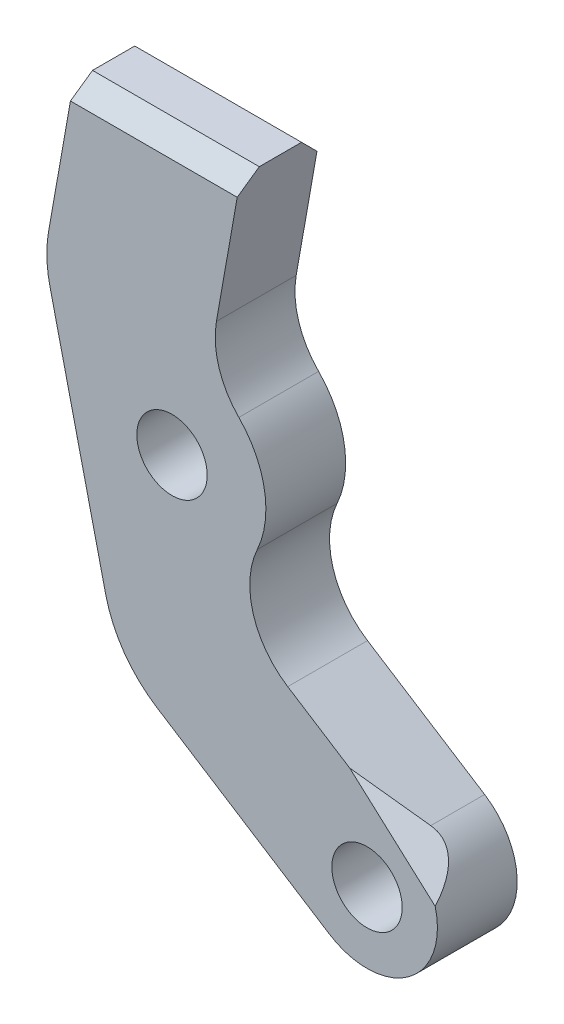
SolidWorks part; units mm, degrees
material "普通碳钢"
ref_plane "前视" through (0, 0, 0) normal (0, 0, 1) x (1, 0, 0)
ref_plane "上视" through (0, 0, 0) normal (0, 1, 0) x (1, 0, 0)
ref_plane "右视" through (0, 0, 0) normal (1, 0, 0) x (0, 0, -1)
sketch "草图1" plane through (0, 0, 0) normal (0, 0, 1) x (1, 0, 0)
  line L0 (-57.5777, 0) -> (30, 0) construction
  line L1 (0, 0) -> (0, -37.5217) construction
  line L2 (-125, 235) -> (-53.92, 235)
  line L3 (-125, 235) -> (-137.4861, 164.188)
  line L5 (-137.4861, 164.188) -> (-106.7282, 32.481)
  line L6 (-69.9882, 80.2135) -> (16.1306, 25.2944)
  line L8 (-106.7282, 32.481) -> (-16.1306, -25.2944)
  line L9 (50, 0) -> (-50, 0) construction
  line L10 (0, -50) -> (0, 50) construction
  line L12 (-53.92, 235) -> (-68.0184, 155.0438)
  arc A0 (-69.9882, 80.2135) -> (-58.4297, 86.5217) centre (-83.11, 118) ccw
  arc A2 (-58.4297, 86.5217) -> (-68.0184, 155.0438) centre (-83.11, 118) ccw
  arc A3 (-16.1306, -25.2944) -> (16.1306, 25.2944) centre (0, 0) ccw
  dimension "D10" = 53.92
  dimension "D7" = 164.188
  dimension "D4" = 30
  dimension "D5" = 40
  dimension "D2" = 235
  dimension "D3" = 70.0001
  dimension "D6" = 100
  dimension "D8" = 118
  dimension "D9" = 83.11
  dimension "D11" = 32.481
  dimension "D12" = 106.7282
  dimension "D13" = 137.4861
extrude "凸台-拉伸1" add sketch "草图1" along normal blind 34
chamfer "倒角1" distance 8 angle 45 2 edges at (-89.46, 235, 0) (-89.46, 235, 34)
sketch "草图2" plane through (0, 0, 0) normal (0, 0, -1) x (-1, 0, 0)
  line L1 (53.92, 235) -> (125, 235) construction
  line L2 (126.4106, 227) -> (137.4861, 164.188) construction
  line L3 (126.4106, 227) -> (137.4861, 164.188) construction
  circle A0 centre (0.0084, 0) radius 15
  circle A1 centre (83.1206, 118) radius 15
  dimension "D1" = 30
  dimension "D2" = 30
  dimension "D3" = 163.9
  dimension "D4" = 117
  dimension "D5" = 61.56
  dimension "D6" = 235
extrude "切除-拉伸1" cut sketch "草图2" against normal through all
fillet "圆角2" radius 35 2 edges at (-69.9882, 80.2135, 17) (-68.0184, 155.0438, 17)
fillet "圆角4" radius 50 2 edges at (-106.7282, 32.481, 17) (-137.4861, 164.188, 17)
ref_plane "基准面3" through (0, 0, 0) normal (0.7431, -0.6691, 0) x (0, 0, -1)
sketch "草图4" plane through (0, 0, 0) normal (0.7431, -0.6691, 0) x (0, 0, -1)
  line L0 (-34, 25) -> (-22, 30)
  line L1 (-34, 30) -> (-34, -29.5908) construction
  line L2 (-22, 30) -> (-34, 30)
  line L3 (-34, 43.966) -> (-34, 19.3666) construction
  line L4 (-34, 30) -> (-34, 25)
  line L5 (-34, 0) -> (0, 0) construction
  dimension "D1" = 5
  dimension "D2" = 12
  dimension "D3" = 25
extrude "切除-拉伸2" cut sketch "草图4" against normal up to surface and the other way through all up to face at (-44.422, 77.99, 17)
